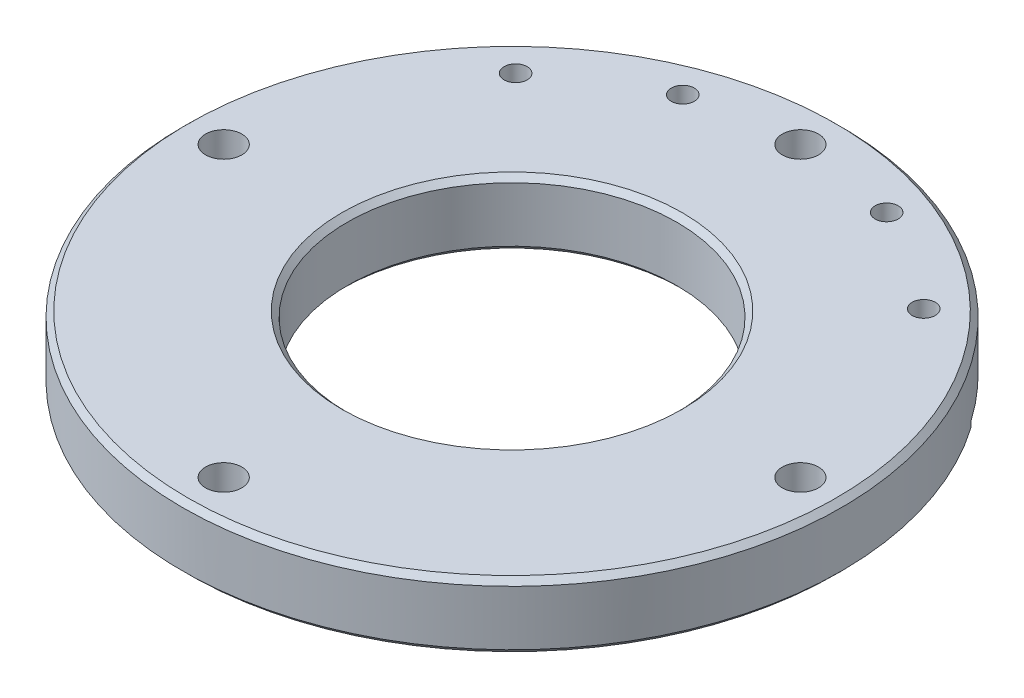
from build123d import *

# Parameters (mm, degrees)
SKETCH1_R                                            = 60
SKETCH1_R_2                                          = 30
BOSS_EXTRUDE1_DEPTH                                  = 6
CHAMFER1_SIZE                                        = 1
HOLE_SIZE_BY_SOCKET_HEAD_CAP_SCREW_TYPE1_D           = 6.6
HOLE_SIZE_BY_SOCKET_HEAD_CAP_SCREW_TYPE1_CBORE_D     = 11
HOLE_SIZE_BY_SOCKET_HEAD_CAP_SCREW_TYPE1_CBORE_DEPTH = 6.8
CUT_EXTRUDE1_START                                   = -2
CUT_EXTRUDE1_DEPTH                                   = 2
FILLET1_R                                            = 2
M5_TAPPED_HOLE1_D                                    = 4.2


with BuildPart() as part:
    # Sketch1 → Boss-Extrude1 (new, symmetric)
    with BuildSketch(Plane(origin=(0, 0, 0), x_dir=(1, 0, 0), z_dir=(0, 1, 0))):
        with Locations(Location((0, 0, 0), (0, 0, 270))):
            Circle(SKETCH1_R)
        with Locations(Location((0, 0, 0), (0, 0, 270))):
            Circle(SKETCH1_R_2, mode=Mode.SUBTRACT)
    extrude(amount=BOSS_EXTRUDE1_DEPTH, both=True)

    # Chamfer1
    chamfer1_edges = [part.edges().sort_by_distance(p)[0] for p in [
        (0, -6, -60),
        (0, 6, -60),
        (0, -6, -30),
        (0, 6, -30),
    ]]
    chamfer(chamfer1_edges, length=CHAMFER1_SIZE)

    # Hole Size by Socket Head Cap Screw Type1 (through all)
    with Locations(Plane(origin=(-41.126423616, -6, 15.006070464), x_dir=(1, 0, 0), z_dir=(0, -1, 0))):
        with Locations((-11.373576384, -15.006070464), (93.626423616, -15.006070464), (41.126423616, -67.506070464), (41.126423616, 37.493929536)):
            CounterBoreHole(HOLE_SIZE_BY_SOCKET_HEAD_CAP_SCREW_TYPE1_D / 2, HOLE_SIZE_BY_SOCKET_HEAD_CAP_SCREW_TYPE1_CBORE_D / 2, HOLE_SIZE_BY_SOCKET_HEAD_CAP_SCREW_TYPE1_CBORE_DEPTH)

    # Sketch4 → Cut-Extrude1 (cut)
    with BuildSketch(Plane.XZ.offset(6).offset(CUT_EXTRUDE1_START)):
        with BuildLine():
            Line((-37.680994037, -26.384516072), (-49.149122657, -34.414586181))
            ThreePointArc((-49.149122657, -34.414586181), (-32.237976501, -50.603486749), (-10.41889066, -59.088465181))
            Line((-10.41889066, -59.088465181), (-7.987816173, -45.301156639))
            ThreePointArc((-7.987816173, -45.301156639), (-24.715781984, -38.796006507), (-37.680994037, -26.384516072))
        make_face()
        with BuildLine():
            Line((7.987816173, -45.301156639), (10.41889066, -59.088465181))
            ThreePointArc((10.41889066, -59.088465181), (32.237976501, -50.603486749), (49.149122657, -34.414586181))
            Line((49.149122657, -34.414586181), (37.680994037, -26.384516072))
            ThreePointArc((37.680994037, -26.384516072), (24.715781984, -38.796006507), (7.987816173, -45.301156639))
        make_face()
    extrude(amount=CUT_EXTRUDE1_DEPTH, mode=Mode.SUBTRACT)

    # Fillet1
    fillet1_edges = [part.edges().sort_by_distance(p)[0] for p in [
        (-37.680994037, -5, -26.384516072),
        (-7.987816173, -5, -45.301156639),
        (7.987816173, -5, -45.301156639),
        (37.680994037, -5, -26.384516072),
    ]]
    fillet(fillet1_edges, radius=FILLET1_R)

    # M5 Tapped Hole1 (through all)
    with Locations(Plane(origin=(0, -4, 0), x_dir=(-1, 0, 0), z_dir=(0, -1, 0))):
        with Locations((37.148191008, 37.802273805), (18.560991207, 49.64362603), (-18.560991207, 49.64362603), (-37.148191008, 37.802273805)):
            Hole(M5_TAPPED_HOLE1_D / 2)


solid = part.part
